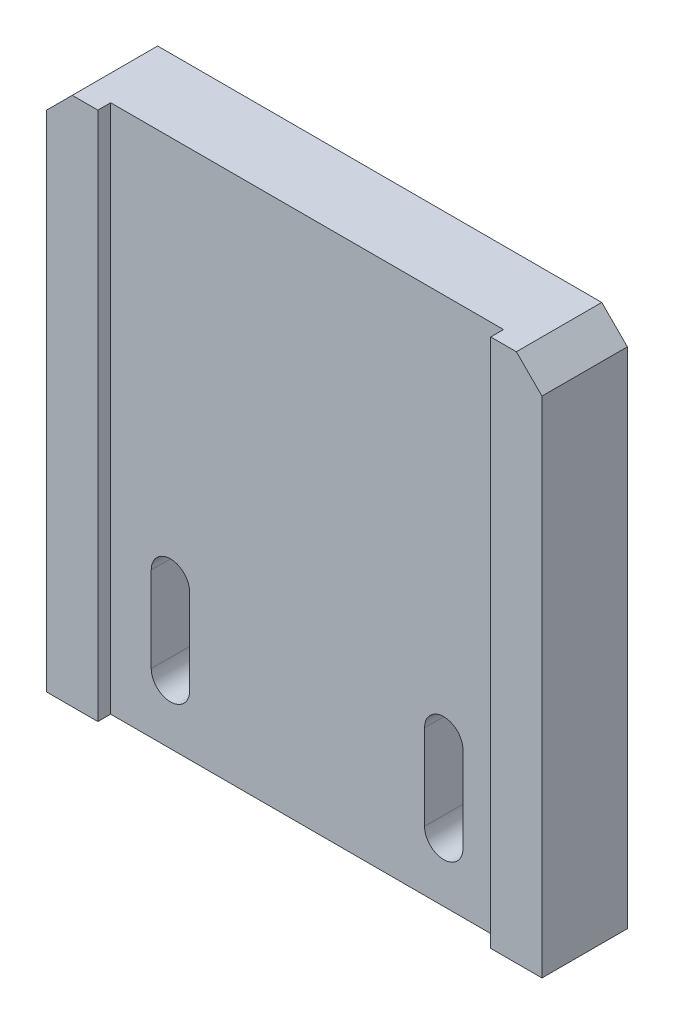
SolidWorks part; units mm, degrees
ref_plane "前视基准面" through (0, 0, 0) normal (0, 0, 1) x (1, 0, 0)
ref_plane "上视基准面" through (0, 0, 0) normal (0, 1, 0) x (1, 0, 0)
ref_plane "右视基准面" through (0, 0, 0) normal (1, 0, 0) x (0, 0, -1)
sketch "草图1" plane through (0, 0, 0) normal (0, 0, 1) x (1, 0, 0)
  line L1 (-29, -31) -> (29, -31)
  line L2 (-29, -31) -> (-29, 31)
  line L3 (-29, 31) -> (29, 31)
  line L4 (29, -31) -> (29, 31)
  line L5 (-29, -31) -> (29, 31) construction
  line L6 (-29, 31) -> (29, -31) construction
  point P0 (0, 0)
  dimension "D1" = 58
  dimension "D2" = 62
extrude "凸台-拉伸1" add sketch "草图1" along normal blind 10
sketch "草图2" plane through (0, 0, 10) normal (0, 0, 1) x (1, 0, 0)
  line L0 (29, 31) -> (-29, 31) construction
  line L1 (-23, -31) -> (23, -31)
  line L2 (-23, -31) -> (-23, 31)
  line L3 (-23, 31) -> (23, 31)
  line L4 (23, -31) -> (23, 31)
  line L5 (-23, -31) -> (23, 31) construction
  line L6 (-23, 31) -> (23, -31) construction
  point P0 (0, 0)
  dimension "D1" = 46
extrude "切除-拉伸1" cut sketch "草图2" against normal blind 1.5
chamfer "倒角1" distance 3 angle 45 2 edges at (-29, 31, 5) (29, 31, 5)
sketch "草图3" plane through (0, 0, 8.5) normal (0, 0, 1) x (1, 0, 0)
  line L0 (-16, -24) -> (-16, -14) construction
  line L1 (-18.25, -24) -> (-18.25, -14)
  line L2 (-13.75, -24) -> (-13.75, -14)
  line L3 (-23, -31) -> (23, -31) construction
  arc A0 (-18.25, -24) -> (-13.75, -24) centre (-16, -24) ccw
  arc A1 (-13.75, -14) -> (-18.25, -14) centre (-16, -14) ccw
  point P2 (-16, -19)
  dimension "D1" = 2.25
  dimension "D2" = 16
  dimension "D3" = 10
  dimension "D4" = 12
extrude "切除-拉伸2" cut sketch "草图3" against normal up to next
mirror "镜向1" about plane through (0, 0, 0) normal (1, 0, 0) of "切除-拉伸2"
